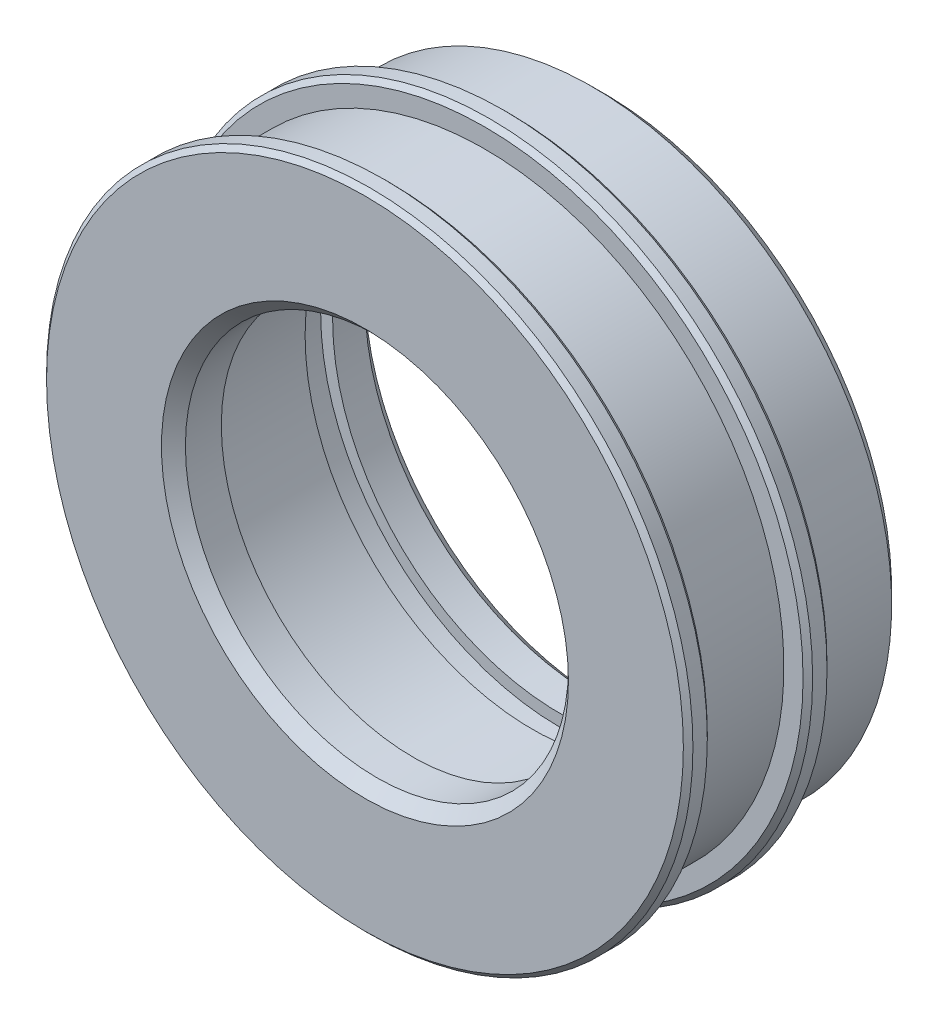
from build123d import *

# Parameters (mm, degrees)
SKETCH_1_R          = 12.5
SKETCH_1_R_2        = 8
EXTRUDE_1_DEPTH     = 4
SKETCH_2_R          = 13.5
SKETCH_2_R_2        = 8
EXTRUDE_2_DEPTH     = 1
EXTRUDE_START       = 1
SKETCH_3_R          = 13.5
SKETCH_3_R_2        = 8
EXTRUDE_3_DEPTH     = 1
SKETCH_4_R          = 9.5
CUT_EXTRUDE_1_DEPTH = 4
EXTRUDE_START_2     = 4
SKETCH_7_R          = 12.5
SKETCH_7_R_2        = 9.5
EXTRUDE_4_DEPTH     = 4
CUT_EXTRUDE_START   = -3
SKETCH_8_R          = 10
SKETCH_8_R_2        = 6
CUT_EXTRUDE_2_DEPTH = 1.15
CHAMFER_1_SIZE      = 0.5
CHAMFER_2_SIZE      = 0.2


with BuildPart() as part:
    # 草图1 → 凸台-拉伸1 (new body)
    with BuildSketch(Plane.XY):
        Circle(SKETCH_1_R)
        Circle(SKETCH_1_R_2, mode=Mode.SUBTRACT)
    extrude(amount=EXTRUDE_1_DEPTH)

    # 草图2 → 凸台-拉伸2 (add)
    with BuildSketch(Plane.XY.offset(4)):
        Circle(SKETCH_2_R)
        Circle(SKETCH_2_R_2, mode=Mode.SUBTRACT)
    extrude(amount=EXTRUDE_2_DEPTH)

    # 草图3 → 凸台-拉伸3 (add)
    with BuildSketch(Plane(origin=(0, 0, 0), x_dir=(-1, 0, 0), z_dir=(0, 0, -1)).offset(EXTRUDE_START)):
        with Locations(Location((0, 0, 0), (0, 0, 180))):
            Circle(SKETCH_3_R)
        Circle(SKETCH_3_R_2, mode=Mode.SUBTRACT)
    extrude(amount=-EXTRUDE_3_DEPTH)

    # 草图4 → 切除-拉伸1 (cut)
    with BuildSketch(Plane(origin=(0, 0, -1), x_dir=(-1, 0, 0), z_dir=(0, 0, -1))):
        Circle(SKETCH_4_R)
    extrude(amount=-CUT_EXTRUDE_1_DEPTH, mode=Mode.SUBTRACT)

    # 草图7 → 凸台-拉伸4 (add)
    with BuildSketch(Plane(origin=(0, 0, -1), x_dir=(-1, 0, 0), z_dir=(0, 0, -1)).offset(EXTRUDE_START_2)):
        Circle(SKETCH_7_R)
        Circle(SKETCH_7_R_2, mode=Mode.SUBTRACT)
    extrude(amount=-EXTRUDE_4_DEPTH)

    # 草图8 → 切除-拉伸2 (cut)
    with BuildSketch(Plane(origin=(0, 0, -5), x_dir=(-1, 0, 0), z_dir=(0, 0, -1)).offset(CUT_EXTRUDE_START)):
        Circle(SKETCH_8_R)
        Circle(SKETCH_8_R_2, mode=Mode.SUBTRACT)
    extrude(amount=CUT_EXTRUDE_2_DEPTH, mode=Mode.SUBTRACT)

    # 倒角1
    chamfer_1_edges = [part.edges().sort_by_distance(p)[0] for p in [
        (-8, 0, 5),
        (12.5, 0, -5),
        (9.5, 0, -5),
    ]]
    chamfer(chamfer_1_edges, length=CHAMFER_1_SIZE)

    # 倒角2
    chamfer_2_edges = [part.edges().sort_by_distance(p)[0] for p in [
        (-13.5, 0, 4),
        (-13.5, 0, -1),
        (-13.5, 0, 0),
        (-13.5, 0, 5),
    ]]
    chamfer(chamfer_2_edges, length=CHAMFER_2_SIZE)


solid = part.part
